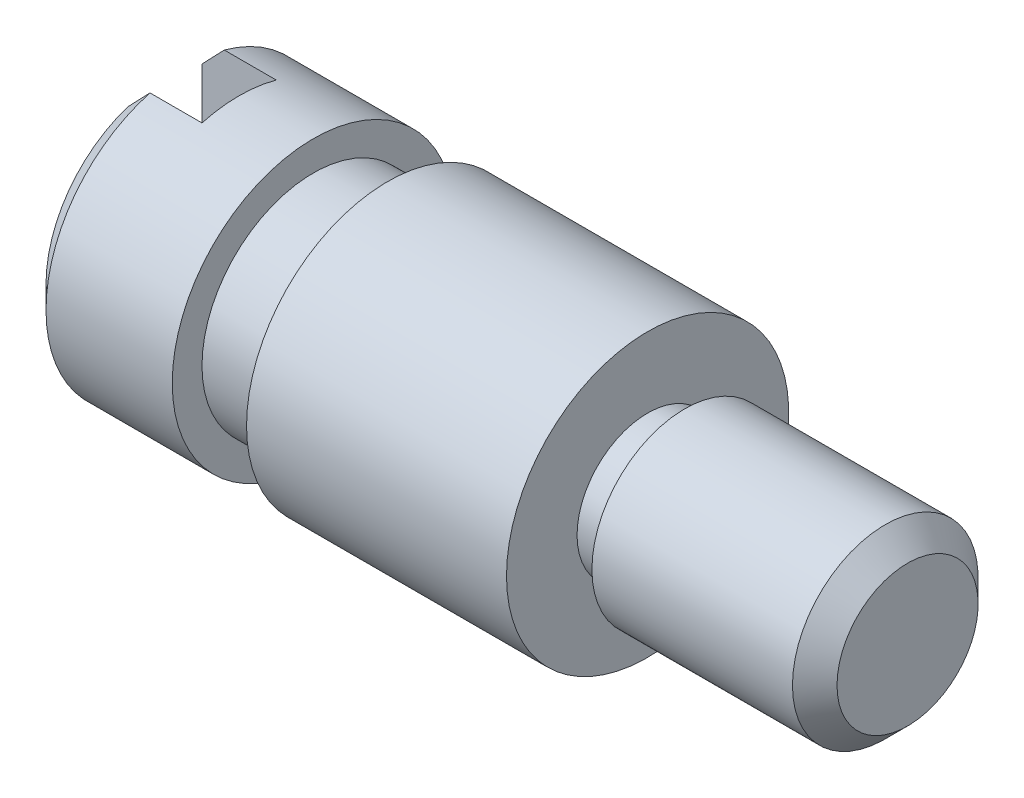
from build123d import *

# Parameters (mm, degrees)
SKETCH2_W          = 1
SKETCH2_H          = 6.77698326
CUT_EXTRUDE1_DEPTH = 1


with BuildPart() as part:
    # Sketch1 → Revolve1 (revolve)
    with BuildSketch(Plane(origin=(0, 0, 0), x_dir=(1, 0, 0), z_dir=(0, 1, 0)), mode=Mode.PRIVATE) as revolve1_sk:
        Polygon((0, 0), (-10, 0), (-10, 1.6), (-9.7, 1.9), (-8, 1.9), (-8, 1.5), (-7, 1.5), (-7, 1.9), (-3.5, 1.9), (-3.5, 0.95), (-3, 0.95), (-3, 1.25), (-0.3, 1.25), (0, 0.95), align=None)
    revolve(revolve1_sk.sketch.rotate(Axis((0, 0, 0), (1, 0, 0)), 180), axis=Axis((0, 0, 0), (1, 0, 0)))

    # Sketch2 → Cut-Extrude1 (cut)
    with BuildSketch(Plane.ZY.offset(10)):
        Rectangle(SKETCH2_W, SKETCH2_H)
    extrude(amount=-CUT_EXTRUDE1_DEPTH, mode=Mode.SUBTRACT)


solid = part.part
